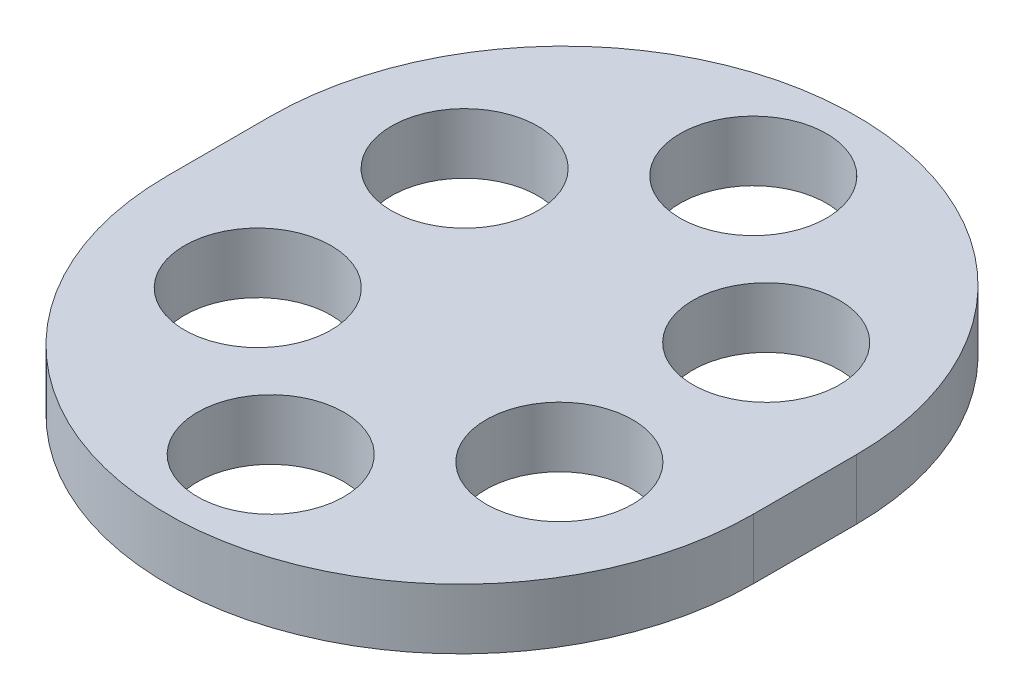
SolidWorks part; units mm, degrees
material "45"
ref_plane "前视基准面" through (0, 0, 0) normal (0, 0, 1) x (1, 0, 0)
ref_plane "上视基准面" through (0, 0, 0) normal (0, 1, 0) x (1, 0, 0)
ref_plane "右视基准面" through (0, 0, 0) normal (1, 0, 0) x (0, 0, -1)
sketch "草图1" plane through (0, 0, 0) normal (0, 1, 0) x (1, 0, 0)
  line L0 (0, 6) -> (0, -6) construction
  line L5 (0, 0) -> (34, 0) construction
  line L6 (34, -6) -> (34, 6)
  line L7 (-34, -6) -> (-34, 6)
  arc A0 (34, 6) -> (-34, 6) centre (0, 6) ccw
  arc A1 (34, -6) -> (-34, -6) centre (0, -6) cw
  circle A2 centre (0, 28) radius 8.5
  circle A3 centre (-17.5, 12) radius 8.5
  circle A4 centre (17.5, 12) radius 8.5
  circle A5 centre (17.5, -12) radius 8.5
  circle A6 centre (-17.5, -12) radius 8.5
  circle A7 centre (0, -28) radius 8.5
  point P4 (0, 40)
  point P11 (-34, 0)
  point P12 (0, -40)
  dimension "D1" = 34
  dimension "D5" = 17
  dimension "D7" = 24
  dimension "D8" = 35
  dimension "D2" = 34
  dimension "D3" = 6
  dimension "D4" = 80
  dimension "D6" = 56
extrude "凸台-拉伸1" add sketch "草图1" along normal blind 7
